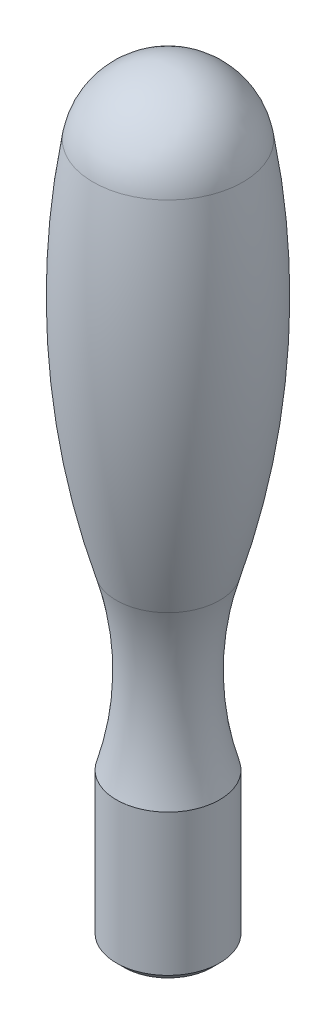
from build123d import *


with BuildPart() as part:
    # Sketch1 → Revolve1 (revolve)
    with BuildSketch(Plane.XY, mode=Mode.PRIVATE) as revolve1_sk:
        with BuildLine():
            Line((-103.1, 87.762990915), (-103.1, 97.076733695))
            ThreePointArc((-103.1, 97.076733695), (-103.925983982, 102.765064712), (-103.1, 108.453395729))
            ThreePointArc((-103.1, 108.453395729), (-100.934781518, 120.679460223), (-101.567145595, 133.079659404))
            ThreePointArc((-101.567145595, 133.079659404), (-103.266066052, 136.076345242), (-106.5, 137.262990915))
            Line((-106.5, 137.262990915), (-106.5, 87.262990915))
            Line((-106.5, 87.262990915), (-103.6, 87.262990915))
            Line((-103.6, 87.262990915), (-103.1, 87.762990915))
        make_face()
    revolve(revolve1_sk.sketch.rotate(Axis((-106.5, 85.3, 0), (0, 1, 0)), 90), axis=Axis((-106.5, 85.3, 0), (0, 1, 0)))


solid = part.part
